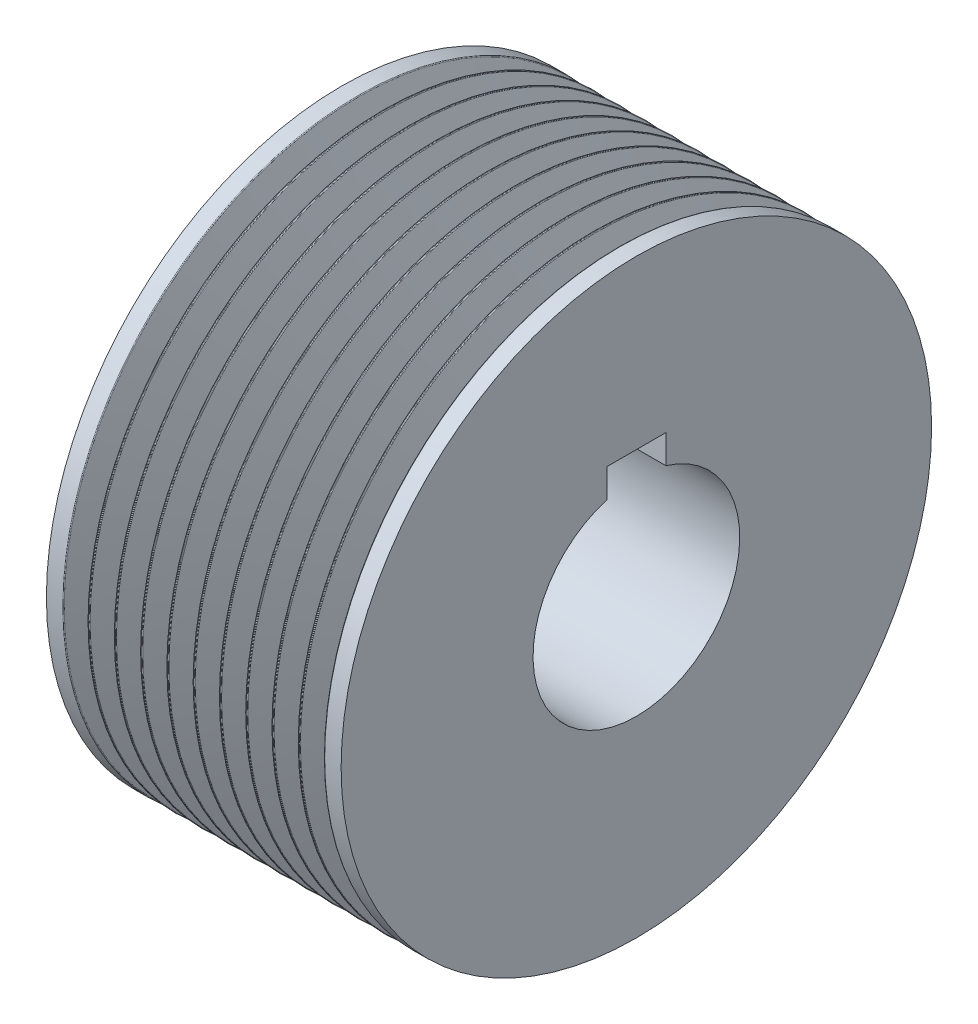
SolidWorks part; units mm, degrees
material "普通碳钢"
ref_plane "Front Plane" through (0, 0, 0) normal (0, 0, 1) x (1, 0, 0)
ref_plane "Top Plane" through (0, 0, 0) normal (0, 1, 0) x (1, 0, 0)
ref_plane "Right Plane" through (0, 0, 0) normal (1, 0, 0) x (0, 0, -1)
sketch "Sketch1" plane through (0, 0, 0) normal (0, 0, 1) x (1, 0, 0)
  line L0 (-0.12, -0.1) -> (-0.12, -40)
  line L1 (0, 0) -> (2.2, 0)
  line L2 (0, 0) -> (0, -40)
  line L4 (2.2, 0) -> (2.2, -40)
  line L5 (0, 0) -> (2.2, -40) construction
  line L6 (0, -40) -> (2.2, 0) construction
  line L7 (-1.5144, -3.45) -> (-1.9744, -3.45)
  line L8 (-2.2093, -3.2855) -> (-3.3812, -0.0658)
  line L9 (-3.4751, 0) -> (-3.5653, 0)
  line L10 (-3.6591, -0.0656) -> (-4.8396, -3.286)
  line L11 (-1.7444, 2.0998) -> (-1.7444, -5.2762) construction
  line L12 (-0.02, 0) -> (0, 0)
  line L13 (-37.73, -40) -> (2.2, -40)
  line L14 (-0.12, -0.1) -> (-1.2794, -3.2855)
  line L15 (-5.0744, -3.45) -> (-5.5344, -3.45)
  line L16 (-5.7693, -3.2855) -> (-6.9412, -0.0658)
  line L17 (-7.0351, 0) -> (-7.1253, 0)
  line L18 (-7.2191, -0.0656) -> (-8.3994, -3.2855)
  line L19 (-8.6344, -3.45) -> (-9.0944, -3.45)
  line L20 (-9.3293, -3.2855) -> (-10.5012, -0.0658)
  line L21 (-10.5951, 0) -> (-10.6853, 0)
  line L22 (-10.7791, -0.0656) -> (-11.9594, -3.2855)
  line L23 (-12.1944, -3.45) -> (-12.6544, -3.45)
  line L24 (-12.8893, -3.2855) -> (-14.0612, -0.0658)
  line L25 (-14.1551, 0) -> (-14.2453, 0)
  line L26 (-14.3391, -0.0656) -> (-15.5194, -3.2855)
  line L27 (-15.7544, -3.45) -> (-16.2144, -3.45)
  line L28 (-16.4493, -3.2855) -> (-17.6212, -0.0658)
  line L29 (-17.7151, 0) -> (-17.8053, 0)
  line L30 (-17.8991, -0.0656) -> (-19.0794, -3.2855)
  line L31 (-19.3144, -3.45) -> (-19.7744, -3.45)
  line L32 (-20.0093, -3.2855) -> (-21.1812, -0.0658)
  line L33 (-21.2751, 0) -> (-21.3653, 0)
  line L34 (-21.4591, -0.0656) -> (-22.6394, -3.2855)
  line L35 (-22.8744, -3.45) -> (-23.3344, -3.45)
  line L36 (-23.5693, -3.2855) -> (-24.7412, -0.0658)
  line L37 (-24.8351, 0) -> (-24.9253, 0)
  line L38 (-25.0191, -0.0656) -> (-26.1994, -3.2855)
  line L39 (-26.4344, -3.45) -> (-26.8944, -3.45)
  line L40 (-27.1293, -3.2855) -> (-28.3012, -0.0658)
  line L41 (-28.3951, 0) -> (-28.4853, 0)
  line L42 (-28.5791, -0.0656) -> (-29.7594, -3.2855)
  line L43 (-29.9944, -3.45) -> (-30.4544, -3.45)
  line L44 (-30.6893, -3.2855) -> (-31.8612, -0.0658)
  line L45 (-31.9551, 0) -> (-32.0453, 0)
  line L46 (-32.1391, -0.0656) -> (-33.3194, -3.2855)
  line L47 (-33.5544, -3.45) -> (-34.0144, -3.45)
  line L48 (-34.2493, -3.2855) -> (-35.4101, -0.0962)
  line L51 (-17.765, -2.3197) -> (-17.765, -6.9133) construction
  line L52 (-35.53, -40) -> (-37.73, 0) construction
  line L53 (-35.53, 0) -> (-37.73, -40) construction
  line L54 (-35.51, 0) -> (-35.53, 0)
  line L55 (-37.73, 0) -> (-37.73, -40)
  line L56 (-35.53, 0) -> (-35.53, -40)
  line L57 (-35.53, 0) -> (-37.73, 0)
  line L58 (-35.41, -0.1) -> (-35.41, -40)
  line L59 (-35.6991, -0.0656) -> (-36.8796, -3.286) [skipped]
  line L60 (-35.5151, 0) -> (-35.6053, 0) [skipped]
  arc A0 (-0.12, -0.1) -> (-0.02, 0) centre (-0.02, -0.1) cw
  arc A1 (-2.2093, -3.2855) -> (-1.9744, -3.45) centre (-1.9744, -3.2) ccw
  arc A2 (-1.2794, -3.2855) -> (-1.5144, -3.45) centre (-1.5144, -3.2) cw
  arc A3 (-3.3812, -0.0658) -> (-3.4751, 0) centre (-3.4751, -0.1) ccw
  arc A4 (-3.5653, 0) -> (-3.6591, -0.0656) centre (-3.5653, -0.1) ccw
  arc A5 (-4.8396, -3.286) -> (-5.0744, -3.45) centre (-5.0744, -3.2) cw
  arc A6 (-5.7693, -3.2855) -> (-5.5344, -3.45) centre (-5.5344, -3.2) ccw
  arc A7 (-6.9412, -0.0658) -> (-7.0351, 0) centre (-7.0351, -0.1) ccw
  arc A8 (-7.1253, 0) -> (-7.2191, -0.0656) centre (-7.1253, -0.1) ccw
  arc A9 (-8.3994, -3.2855) -> (-8.6344, -3.45) centre (-8.6344, -3.2) cw
  arc A10 (-9.3293, -3.2855) -> (-9.0944, -3.45) centre (-9.0944, -3.2) ccw
  arc A11 (-10.5012, -0.0658) -> (-10.5951, 0) centre (-10.5951, -0.1) ccw
  arc A12 (-10.6853, 0) -> (-10.7791, -0.0656) centre (-10.6853, -0.1) ccw
  arc A13 (-11.9594, -3.2855) -> (-12.1944, -3.45) centre (-12.1944, -3.2) cw
  arc A14 (-12.8893, -3.2855) -> (-12.6544, -3.45) centre (-12.6544, -3.2) ccw
  arc A15 (-14.0612, -0.0658) -> (-14.1551, 0) centre (-14.1551, -0.1) ccw
  arc A16 (-14.2453, 0) -> (-14.3391, -0.0656) centre (-14.2453, -0.1) ccw
  arc A17 (-15.5194, -3.2855) -> (-15.7544, -3.45) centre (-15.7544, -3.2) cw
  arc A18 (-16.4493, -3.2855) -> (-16.2144, -3.45) centre (-16.2144, -3.2) ccw
  arc A19 (-17.6212, -0.0658) -> (-17.7151, 0) centre (-17.7151, -0.1) ccw
  arc A20 (-17.8053, 0) -> (-17.8991, -0.0656) centre (-17.8053, -0.1) ccw
  arc A21 (-19.0794, -3.2855) -> (-19.3144, -3.45) centre (-19.3144, -3.2) cw
  arc A22 (-20.0093, -3.2855) -> (-19.7744, -3.45) centre (-19.7744, -3.2) ccw
  arc A23 (-21.1812, -0.0658) -> (-21.2751, 0) centre (-21.2751, -0.1) ccw
  arc A24 (-21.3653, 0) -> (-21.4591, -0.0656) centre (-21.3653, -0.1) ccw
  arc A25 (-22.6394, -3.2855) -> (-22.8744, -3.45) centre (-22.8744, -3.2) cw
  arc A26 (-23.5693, -3.2855) -> (-23.3344, -3.45) centre (-23.3344, -3.2) ccw
  arc A27 (-24.7412, -0.0658) -> (-24.8351, 0) centre (-24.8351, -0.1) ccw
  arc A28 (-24.9253, 0) -> (-25.0191, -0.0656) centre (-24.9253, -0.1) ccw
  arc A29 (-26.1994, -3.2855) -> (-26.4344, -3.45) centre (-26.4344, -3.2) cw
  arc A30 (-27.1293, -3.2855) -> (-26.8944, -3.45) centre (-26.8944, -3.2) ccw
  arc A31 (-28.3012, -0.0658) -> (-28.3951, 0) centre (-28.3951, -0.1) ccw
  arc A32 (-28.4853, 0) -> (-28.5791, -0.0656) centre (-28.4853, -0.1) ccw
  arc A33 (-29.7594, -3.2855) -> (-29.9944, -3.45) centre (-29.9944, -3.2) cw
  arc A34 (-30.6893, -3.2855) -> (-30.4544, -3.45) centre (-30.4544, -3.2) ccw
  arc A35 (-31.8612, -0.0658) -> (-31.9551, 0) centre (-31.9551, -0.1) ccw
  arc A36 (-32.0453, 0) -> (-32.1391, -0.0656) centre (-32.0453, -0.1) ccw
  arc A37 (-33.3194, -3.2855) -> (-33.5544, -3.45) centre (-33.5544, -3.2) cw
  arc A38 (-34.2493, -3.2855) -> (-34.0144, -3.45) centre (-34.0144, -3.2) ccw
  arc A41 (-35.41, -0.1) -> (-35.51, 0) centre (-35.51, -0.1) ccw
  arc A42 (-35.6053, 0) -> (-35.6991, -0.0656) centre (-35.6053, -0.1) ccw [skipped]
  arc A43 (-35.4212, -0.0658) -> (-35.5151, 0) centre (-35.5151, -0.1) ccw [skipped]
  point P4 (1.1, -20)
  point P17 (-0.12, 0)
  point P18 (-1.7444, -3.45)
  point P27 (-3.4051, 0)
  point P30 (-3.6351, 0)
  point P148 (-35.41, 0)
  point P149 (-36.63, -20)
  dimension "D3" = 0.1
  dimension "D7" = 0.25
  dimension "D11" = 0.1
  dimension "D1" = 2.2
  dimension "D2" = 0.12
  dimension "D4" = 40
  dimension "D5" = 0.23
  dimension "D6" = 110
  dimension "D8" = 0.46
  dimension "D9" = 110
  dimension "D10" = 3.45
  dimension "D13" = 39.93
  dimension "D12" = 10
revolve "Revolve1" add sketch "Sketch1" angle 360 about L13
sketch "Sketch2" plane through (2.2, 0, 0) normal (1, 0, 0) x (0, 0, -1)
  line L0 (0, 0) -> (0, -80) construction
  line L1 (-40, -40) -> (40, -40) construction
  line L3 (-4, -22.7) -> (4, -22.7)
  line L4 (-4, -22.7) -> (-4, -26.5836)
  line L6 (4, -22.7) -> (4, -26.5836)
  circle A0 centre (0, -40) radius 40 construction
  arc A1 (-4, -26.5836) -> (4, -26.5836) centre (0, -40) ccw
  dimension "D1" = 28
  dimension "D2" = 17.3
  dimension "D3" = 8
extrude "Cut-Extrude1" cut sketch "Sketch2" against normal through all
